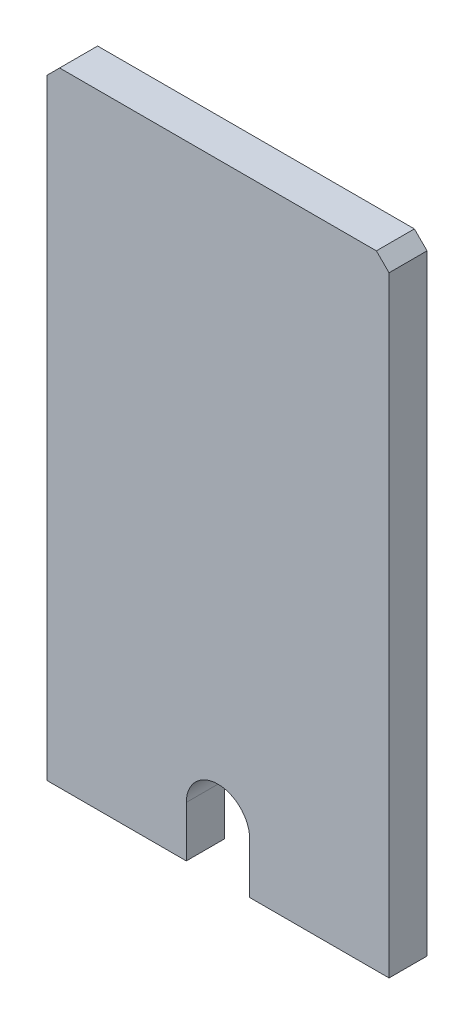
from build123d import *

# Parameters (mm, degrees)
BOSS_EXTRUDE1_DEPTH = 30


with BuildPart() as part:
    # Sketch1 → Boss-Extrude1 (new body)
    with BuildSketch(Plane.XY):
        with BuildLine():
            Line((110, 0), (110, 40))
            ThreePointArc((110, 40), (135, 65), (160, 40))
            Line((160, 40), (160, 0))
            Line((160, 0), (270, 0))
            Line((270, 0), (270, 482))
            Line((270, 482), (260, 492))
            Line((260, 492), (10, 492))
            Line((10, 492), (0, 482))
            Line((0, 482), (0, 0))
            Line((0, 0), (110, 0))
        make_face()
    extrude(amount=BOSS_EXTRUDE1_DEPTH)


solid = part.part
